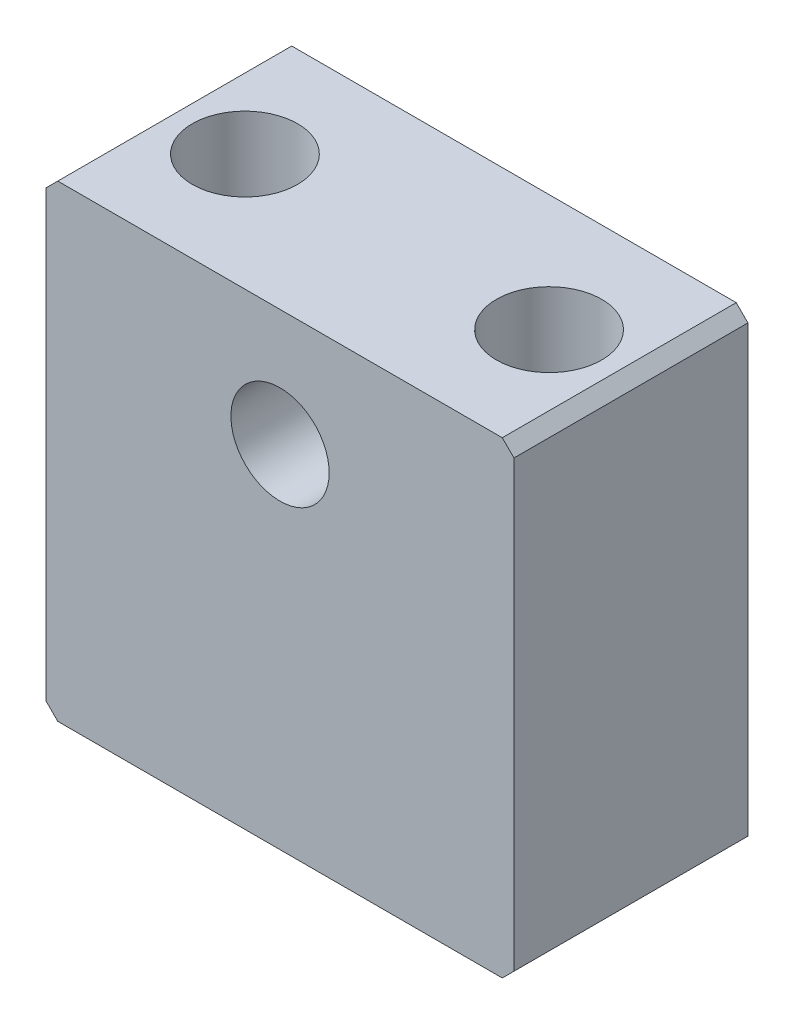
from build123d import *

# Parameters (mm, degrees)
SKETCH1_W            = 20
SKETCH1_H            = 10
BOSS_EXTRUDE1_DEPTH  = 10
M5_TAPPED_HOLE1_D    = 4.2
M4_CLEARANCE_HOLE1_D = 4.5
CHAMFER1_SIZE        = 0.5


with BuildPart() as part:
    # Sketch1 → Boss-Extrude1 (new, symmetric)
    with BuildSketch(Plane(origin=(0, 0, 0), x_dir=(1, 0, 0), z_dir=(0, 1, 0))):
        Rectangle(SKETCH1_W, SKETCH1_H)
    extrude(amount=BOSS_EXTRUDE1_DEPTH, both=True)

    # M5 Tapped Hole1 (through all)
    with Locations(Plane.XY.offset(5)):
        with Locations((0, 5)):
            Hole(M5_TAPPED_HOLE1_D / 2)

    # M4 Clearance Hole1 (through all)
    with Locations(Plane(origin=(0, 10, 0), x_dir=(1, 0, 0), z_dir=(0, 1, 0))):
        with Locations((6.5, 0), (-6.5, 0)):
            Hole(M4_CLEARANCE_HOLE1_D / 2)

    # Chamfer1
    chamfer1_edges = [part.edges().sort_by_distance(p)[0] for p in [
        (-10, 10, 0),
        (10, 10, 0),
        (-10, -10, 0),
        (10, -10, 0),
    ]]
    chamfer(chamfer1_edges, length=CHAMFER1_SIZE)


solid = part.part
